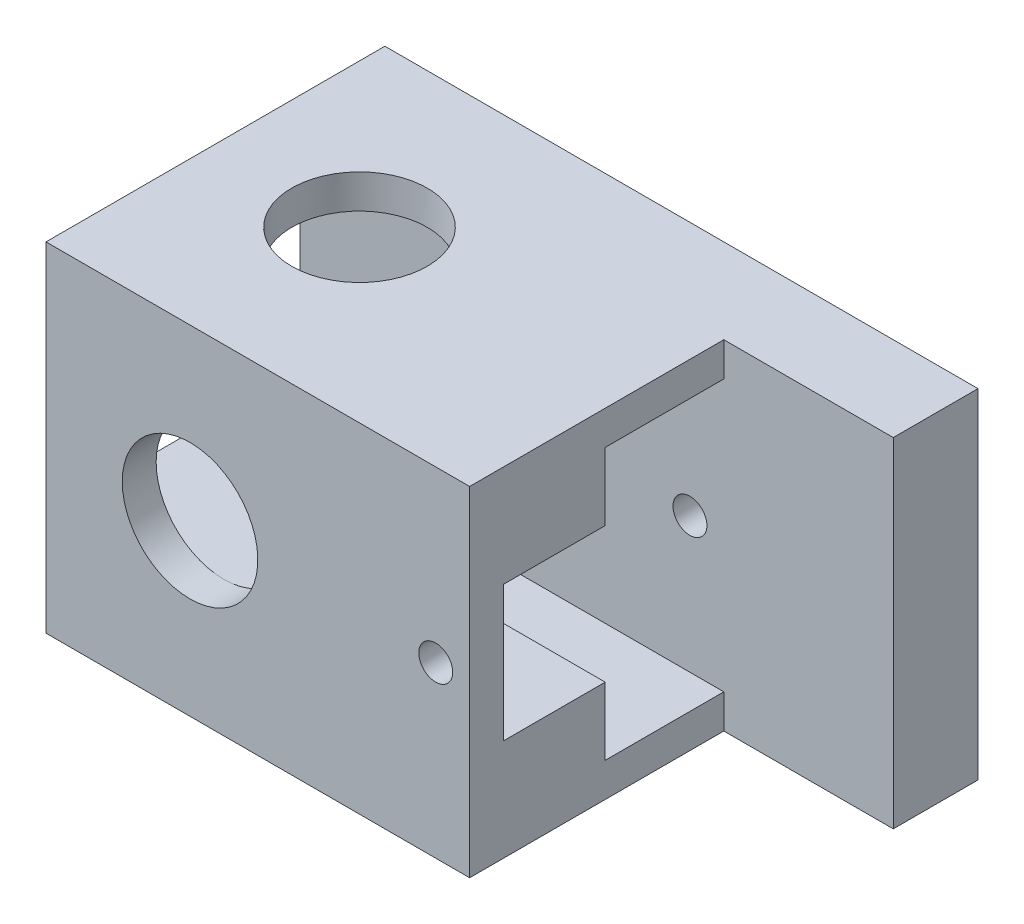
from build123d import *

# Parameters (mm, degrees)
BOSS_EXTRUDE1_DEPTH     = 20
CUT_EXTRUDE1_DEPTH      = 46
CUT_EXTRUDE1_DEPTH_BACK = 46
SKETCH2_R               = 4
SKETCH2_R_2             = 1
CUT_EXTRUDE3_DEPTH      = 46
CUT_EXTRUDE3_DEPTH_BACK = 46
SKETCH5_R               = 4
CUT_EXTRUDE4_DEPTH      = 38.749172176


with BuildPart() as part:
    # Sketch1 → Boss-Extrude1 (new body)
    with BuildSketch(Plane(origin=(0, 0, 0), x_dir=(1, 0, 0), z_dir=(0, 1, 0))):
        Polygon((0, 0), (25, 0), (25, 15), (35, 15), (35, 20), (0, 20), align=None)
    extrude(amount=BOSS_EXTRUDE1_DEPTH)

    # Sketch2 → Cut-Extrude1 (cut, two sides: drawn at the far end of the back side and taken through both)
    with BuildSketch(Plane.XY.offset(-CUT_EXTRUDE1_DEPTH_BACK)):
        with Locations((8.5, 10)):
            Circle(SKETCH2_R)
        with Locations((23, 10)):
            Circle(SKETCH2_R_2)
    extrude(amount=CUT_EXTRUDE1_DEPTH + CUT_EXTRUDE1_DEPTH_BACK, mode=Mode.SUBTRACT)

    # Sketch5 → Cut-Extrude3 (cut, two sides: drawn at the far end of the back side and taken through both)
    with BuildSketch(Plane(origin=(0, 20, 0), x_dir=(1, 0, 0), z_dir=(0, 1, 0)).offset(-CUT_EXTRUDE3_DEPTH_BACK)):
        with Locations(Location((8.5, 10, 0), (0, 0, 270))):
            Circle(SKETCH5_R)
    extrude(amount=CUT_EXTRUDE3_DEPTH + CUT_EXTRUDE3_DEPTH_BACK, mode=Mode.SUBTRACT)

    # Sketch6 → Cut-Extrude4 (cut, through all)
    with BuildSketch(Plane(origin=(25, 0, 0), x_dir=(0, 0, -1), z_dir=(1, 0, 0))):
        Polygon((2, 14), (2, 6), (8, 6), (8, 2.004568818), (15, 2.004568818), (15, 17.995431182), (8, 17.995431182), (8, 14), align=None)
    extrude(amount=-CUT_EXTRUDE4_DEPTH, mode=Mode.SUBTRACT)


solid = part.part
